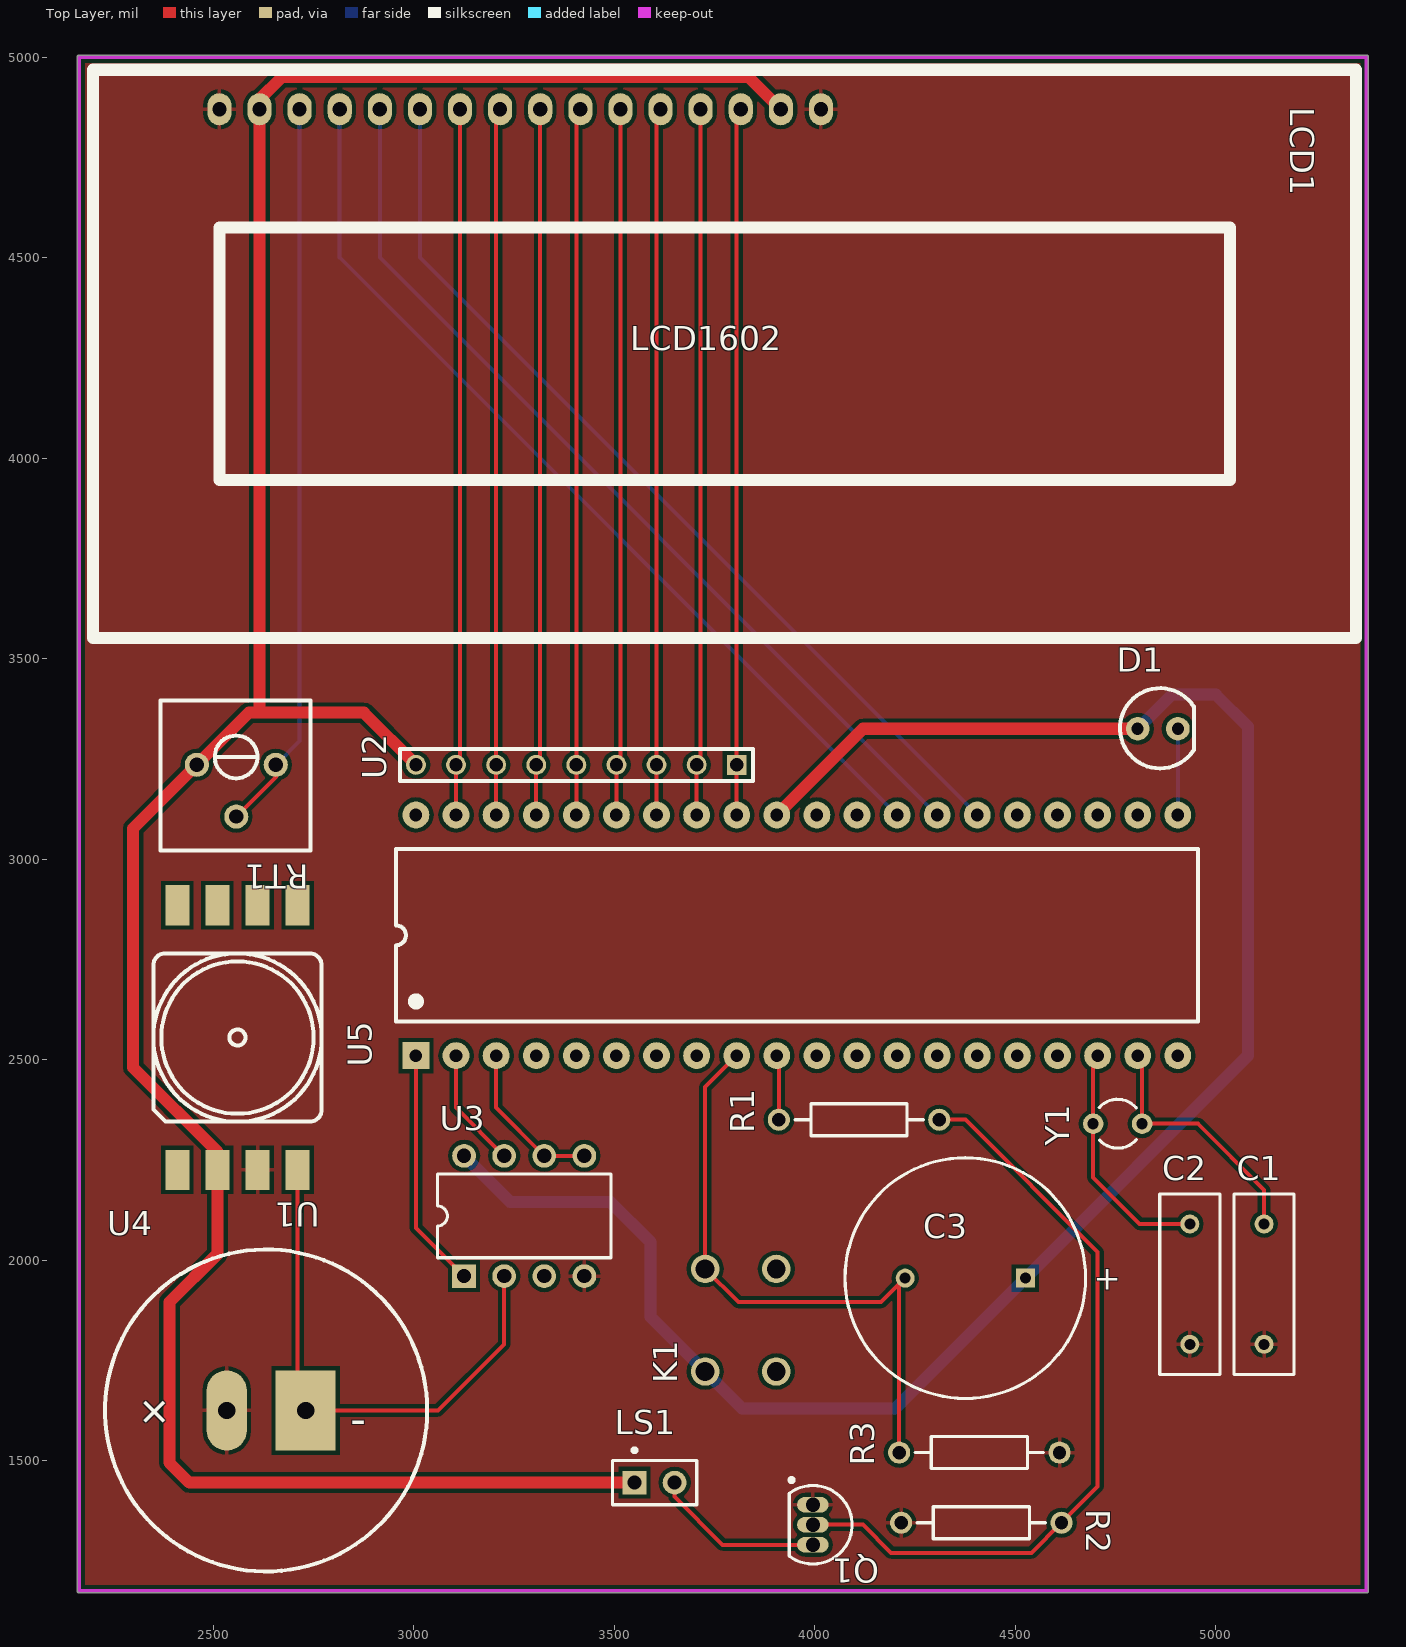
[diagram p0: Top Layer view]
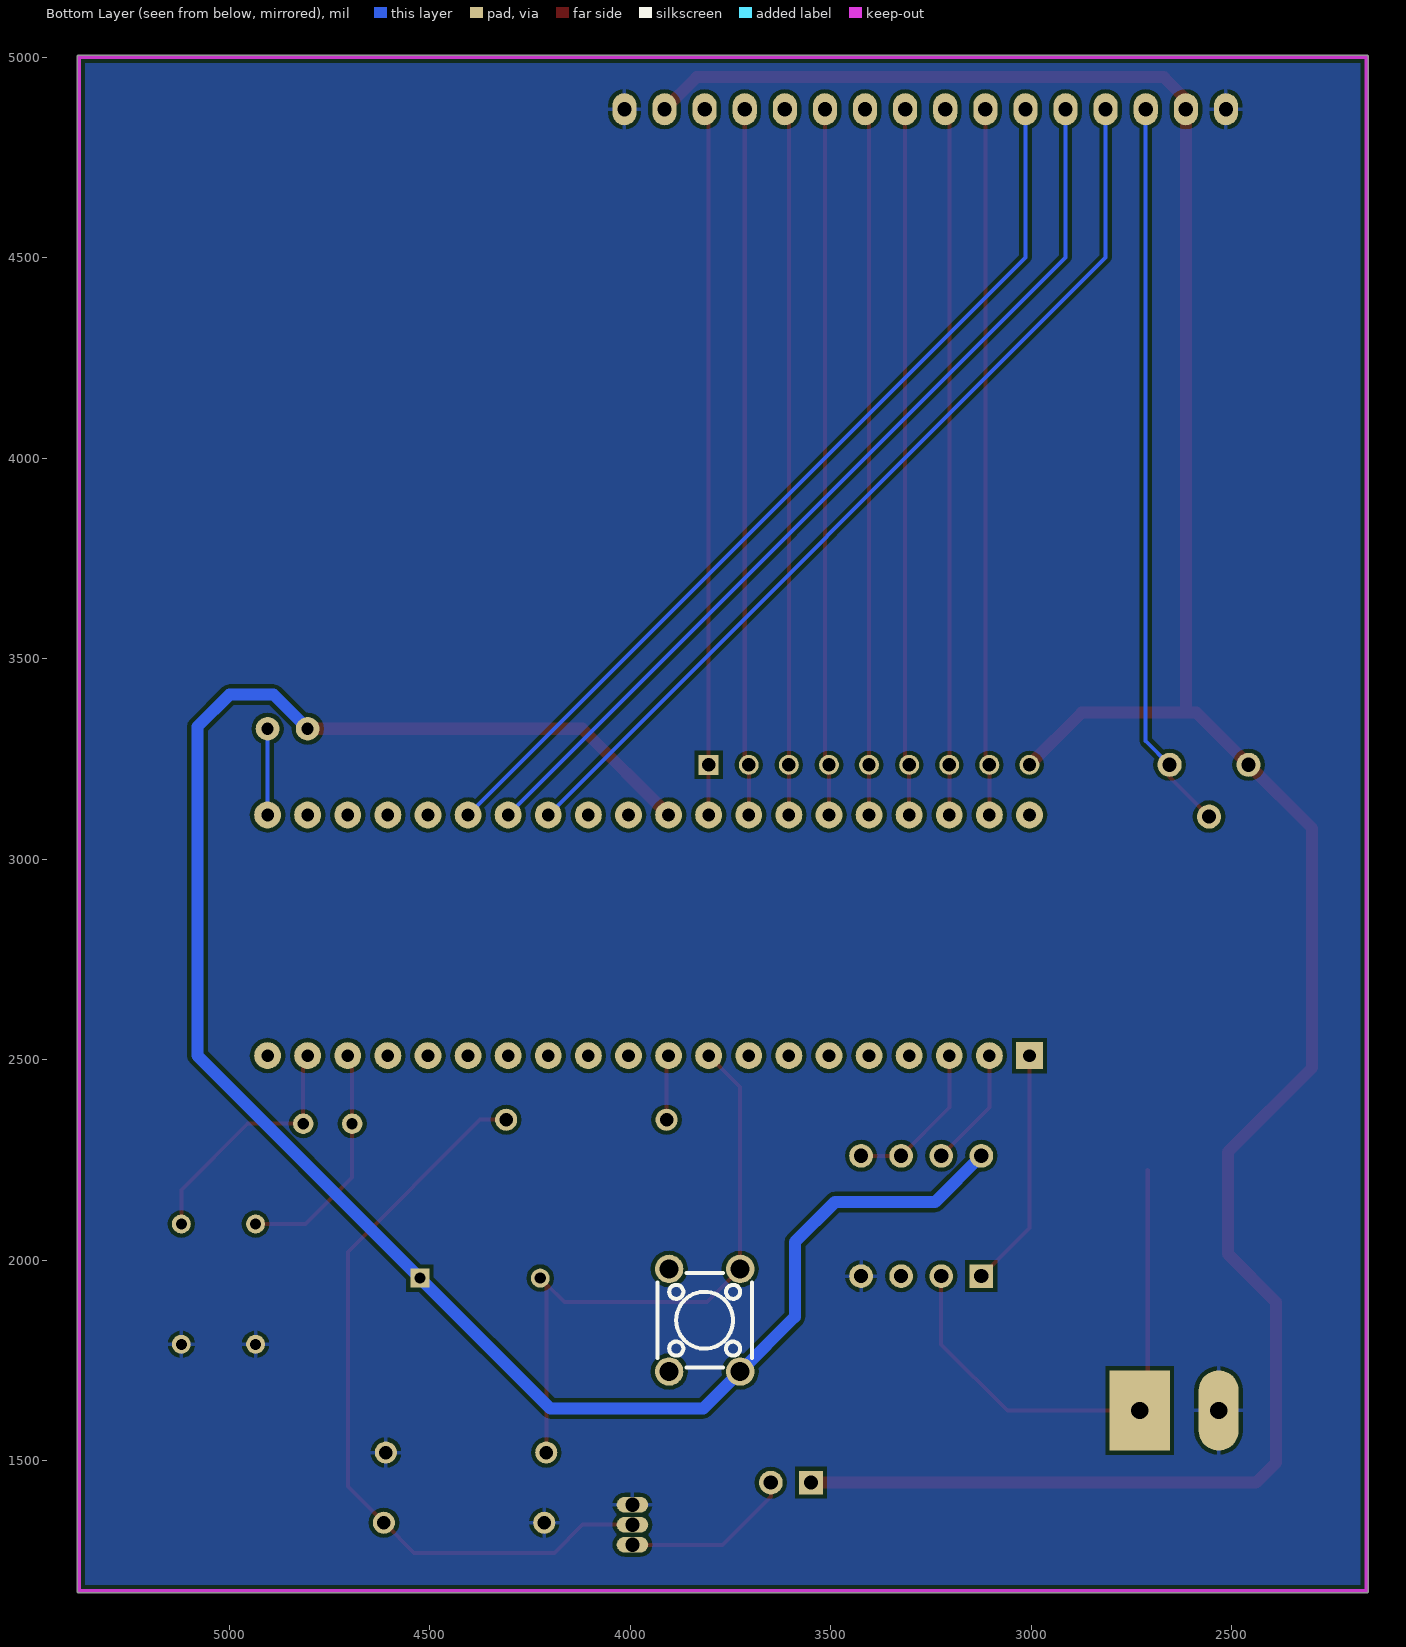
[diagram p1: Bottom Layer view, seen from below]
# Altium PCB MISC84281.PcbDoc
Units mil, origin at the board's own origin, x right, y up, seen from the top; angles counter-clockwise.
Board outline 3220.03 x 3835.03 mil, 2 copper layers (Top Layer, Bottom Layer); 18 components, 32 nets, 111 pads, 0 vias.

## Layer stack, top to bottom (the 12.6 mil dielectric is the usual default, probably not edited)
Top Solder: solder mask 0.4, Solder Resist, Dk 3.5
Top Layer: signal copper 1.4
Dielectric 1: dielectric 12.6, FR-4, Dk 4.8
Bottom Layer: signal copper 1.4
Bottom Solder: solder mask 0.4, Solder Resist, Dk 3.5

## Board outline
2159.99,1175 ccw(c2165,1175) 2165,1169.98 5375,1169.98 ccw(c5375,1175) 5380.02,1175 5380.02,5000 ccw(c5375,5000) 5375,5005.02 2165,5005.02 ccw(c2165,5000) 2159.99,5000

## Design rules (kind name [scope] priority, off if disabled: settings)
Clearance [All] p1: gap=10
MinimumSolderMaskSliver [All] p1: minsoldermaskwidth=0
PolygonConnect [All] p1: connectstyle=Relief reliefconductorwidth=10 reliefentries=4 polygonreliefangle="90 Angle" airgapwidth=10
RoutingVias [All] p1: holewidth=28 width=50 viastyle="Through Hole" minholewidth=28 minwidth=50 maxholewidth=28 maxwidth=50
SilkToSilkClearance [All] p1: silktosilkclearance=0
SilkToSolderMaskClearance [IsPad] p1: minsilkscreentomaskgap=0 clearancetoexposedcopper=TRUE
SolderMaskExpansion [All] p1: expansion=4
Width [All] p1: maxlimit=30 minlimit=10 preferedwidth=10
27 further rules are at their usual default settings.

## Components (designator, comment, footprint, x,y, rotation, side; value= is the part's Value field where it differs from the comment)
C1 "22U" RAD-0.3 5120,1940 r90 top
C2 "22U" RAD-0.3 4935,1940 r90 top
C3 "10UF" RB7.6-15 4375,1955 r0 top
D1 "LED" LED5-BLUE 4805,3325 r0 top
K1 "HH+" 四脚轻触开关 3815,1850 r90 top
LCD1 "LCD1602" LCD1602 2515,4870 r0 top
LS1 "Bell" PIN2 3550,1445 r0 top
Q1 "2N3904" TO-92A 3995,1340 r180 top
R1 "1K" AXIAL-0.4 4110,2350 r180 top
R2 "10K" AXIAL-0.4 4415,1345 r0 top
R3 "10K" AXIAL-0.4 4410,1520 r180 top
RT1 "10K" 电位器 2555,3220 r180 top
U1 "MPXA6115A6U" 482 2560,2555 r270 top
U2 "排阻" paizu 3405,3235 r180 top
U3 "ADC0832" P008 3275,2110 r0 top
U4 "Volts" "CAPACITANCE 1 FARAD 5,5 VOLT" 2631.58,1625 r0 top
U5 "AT89C52" DIP40 3955,2810 r90 top
Y1 "XTAL" R38 4755,2340 r90 top

## Footprints (in the part's own frame and the unit in brackets; to place one, negate y for a bottom-side part, rotate by r counter-clockwise, add the part's x,y. Pads: shape width x height; smd on the part's side, far side on the other; paste and mask are expansions set on the pad)
482 [mil]
  rect 100x60 smd paste+0 mask+2: 1(330,-150) 2(330,-50) 3(330,50) 4(330,150) 5(-330,150) 6(-330,50) 7(-330,-50) 8(-330,-150)
  silkscreen extent -210,-210 210,210
AXIAL-0.4 [mm] "Axial Device, Thru-Hole; 2 Leads; 0.4 in Pin Spacing"
  round 1.4 hole 0.85: 1(-5.08,0) 2(5.08,0)
  silkscreen extent -4.06,-1.02 4.06,1.02
"CAPACITANCE 1 FARAD 5,5 VOLT" [mil]
  rect 150x200 hole 43.31 paste+0 mask+2: 1(98.42,0)
  oval 100x200 hole 43.31 paste+0 mask+2: 2(-98.4,0)
  silkscreen extent -401,-402 402,402
DIP40 [mm]
  rect 1.7x1.7 hole 0.8: 1(-7.62,24.13)
  round 1.7 hole 0.8: 2(-7.62,21.59) 3(-7.62,19.05) 4(-7.62,16.51) 5(-7.62,13.97) 6(-7.62,11.43) 7(-7.62,8.89) 8(-7.62,6.35) 9(-7.62,3.81) 10(-7.62,1.27) 11(-7.62,-1.27) 12(-7.62,-3.81) 13(-7.62,-6.35) 14(-7.62,-8.89) 15(-7.62,-11.43) 16(-7.62,-13.97) 17(-7.62,-16.51) 18(-7.62,-19.05) 19(-7.62,-21.59) 20(-7.62,-24.13) 21(7.62,-24.13) 22(7.62,-21.59) 23(7.62,-19.05) 24(7.62,-16.51) 25(7.62,-13.97) 26(7.62,-11.43) 27(7.62,-8.89) 28(7.62,-6.35) 29(7.62,-3.81) 30(7.62,-1.27) 31(7.62,1.27) 32(7.62,3.81) 33(7.62,6.35) 34(7.62,8.89) 35(7.62,11.43) 36(7.62,13.97) 37(7.62,16.51) 38(7.62,19.05) 39(7.62,21.59) 40(7.62,24.13)
  silkscreen extent -5.46,-25.4 5.46,25.4, body extent -7.91,-26.19 7.65,26.16, height 4.7
LCD1602 [mil]
  oval 60x80 hole 35.43: 1(0,0) 2(100,0) 3(200,0) 4(300,0) 5(400,0) 6(500,0) 7(600,0) 8(700,0) 9(800,0) 10(900,0) 11(1000,0) 12(1100,0) 13(1200,0) 14(1300,0) 15(1400,0) 16(1500,0)
  silkscreen extent -315,-1319 2835,98, body extent -315,-1357 2854,80, height 414
LED5-BLUE [mm]
  round 1.5 hole 0.762: A(0,0) K(2.54,0)
  silkscreen extent -1.12,-2.51 3.56,2.57, body extent -1.58,-2.85 3.77,2.85, height 8.6
P008 [mm] "DIP; 8 Leads; Row Spacing 7.62 mm; Pitch 2.54 mm"
  rect 1.5x1.5 hole 0.9: 1(-3.81,-3.81)
  round 1.5 hole 0.9: 2(-1.27,-3.81) 3(1.27,-3.81) 4(3.81,-3.81) 5(3.81,3.81) 6(1.27,3.81) 7(-1.27,3.81) 8(-3.81,3.81)
  silkscreen extent -5.5,-2.65 5.5,2.65
paizu [mm]
  rect 1.26x1.26 hole 0.84 paste+0 mask+0.051: 1(-10.16,0)
  round 1.26 hole 0.84 paste+0 mask+0.051: 2(-7.62,0) 3(-5.08,0) 4(-2.54,0) 5(0,0) 6(2.54,0) 7(5.08,0) 8(7.62,0) 9(10.16,0)
  silkscreen extent -11.18,-1.02 11.18,1.02
PIN2 [mm] "Photosensitive Diode; 2 Leads"
  rect 1.5x1.5 hole 0.9: 1(0,0)
  round 1.5 hole 0.9: 2(2.54,0)
  silkscreen extent -1.4,-1.4 3.94,2.17
R38 [mm] "Crystal, Thru-Hole; 2 Leads; Body 3.1 x 8.2 mm (Dia.xH)"
  round 1.3 hole 0.7: 1(0,1.55) 2(0,-1.55)
  silkscreen extent -1.55,-1.19 1.55,1.17
RAD-0.3 [mm] "Radial Cap, Thru-Hole; 2 Leads; 0.3 in Pin Spacing"
  round 1.2 hole 0.7: 1(-3.81,0) 2(3.81,0)
  silkscreen extent -5.71,-1.91 5.71,1.91
RB7.6-15 [mm] "Polarized Capacitor (Radial); 2 Leads"
  rect 1.2x1.2 hole 0.7: 1(3.81,0)
  round 1.2 hole 0.7: 2(-3.81,0)
  silkscreen extent -7.62,-7.62 7.62,7.62
TO-92A [mm] "TO, Flat Index; 3 In-Line, Axial Leads; Body Dia. 4.5mm; Leads 0.51 x 0.48 mm (max)"
  oval 2x1 hole 0.9: 1(0,-1.27) 2(0,0) 3(0,1.27)
  silkscreen extent -2.48,-2.95 1.5,2.48, body extent -2.48,-2.5 1.5,2.5, height 6.86
四脚轻触开关 [mm]
  round 1.8 hole 1.2 paste+0 mask+0.102: 1(3.25,2.25) 2(-3.25,2.25) 3(3.25,-2.25) 4(-3.25,-2.25)
电位器 [mil]
  round 60 hole 35.43 paste+0 mask+2: 1(96.41,-15.12) 2(-2.01,114.1) 3(-100.44,-15.12)
  silkscreen extent -187,-175 187,199

## Part data
C1 C2: library part Cap, "Capacitor"
C3: library part "Cap Pol1", "Polarized Capacitor (Radial)"
K1: library part 四脚轻触开关
LS1: "Electrical Bell"
Q1: "NPN General Purpose Amplifier"
R1 R2 R3: library part Res2, "Resistor"
RT1: library part 电位器
U3: "U?"
U5: library part STC89C52
Y1: "Crystal Oscillator"

## Nets (pads, with @x,y where several pads share a name; then routed paths per layer and width w, separated by ;. In a path a pad name is that pad's centre, name@x,y a point inside that pad or via, vN(x,y) a via of type N, cw(c..) or ccw(c..) an arc to the next point about the centre after c; other vN are vias at no path point)
+5: C3.1 D1.A K1.2 U3.8 U5.31 | length 4842.1
  Top Layer w30: U5.31 4120,3325 D1.A
  Bottom Layer w30: U3.8 3240,2145 3490,2145 3590,2045 3590,1858.46 K1.2 3818.46,1630 4200,1630 C3.1 5080,2510 5080,3330 5000,3410 4890,3410 D1.A
GND: C1.1 C2.1 LCD1.1 LCD1.16 Q1.1 R2.1 R3.1 U1.3 U3.4 U4.2
NetC1_2: C1.2 U5.19 Y1.2 | length 631.9
  Top Layer w10: U5.19 4816.02,2498.98 Y1.2 4955,2340 5120,2175 C1.2
NetC2_2: C2.2 U5.18 Y1.1 | length 597.6
  Top Layer w10: U5.18 4693.98,2498.98 Y1.1 4693.98,2206.02 4810,2090 C2.2
NetC3_2: C3.2 K1.1 R3.2 U5.9 | length 1542.4
  Top Layer w10: U5.9 3726.42,2431.42 K1.1 3809.37,1895 4165,1895 C3.2@4210,1940 ; R3.2 C3.2@4210,1940 ; C3.2 C3.2@4210,1940
NetLCD1_3: LCD1.3 RT1.2 RT1.3 | length 1829.5
  Top Layer w10: RT1.2 2655.44,3204.33 RT1.3
  Bottom Layer w10: RT1.3 2715,3294.68 LCD1.3
NetLCD1_4: LCD1.4 U5.28 | length 2335.8
  Bottom Layer w10: LCD1.4 2815,4500 U5.28
NetLCD1_5: LCD1.5 U5.27 | length 2335.8
  Bottom Layer w10: LCD1.5 2915,4500 U5.27
NetLCD1_6: LCD1.6 U5.26 | length 2335.8
  Bottom Layer w10: LCD1.6 3015,4500 U5.26
NetLCD1_7: LCD1.7 U2.8 U5.39 | length 1764.1
  Top Layer w10: U5.39 U2.8 3115,3245 LCD1.7
NetLCD1_8: LCD1.8 U2.7 U5.38 | length 1764.1
  Top Layer w10: U5.38 U2.7 3205,4860 LCD1.8
NetLCD1_9: LCD1.9 U2.6 U5.37 | length 1764.1
  Top Layer w10: U5.37 U2.6 3315,3245 LCD1.9
NetLCD1_10: LCD1.10 U2.5 U5.36 | length 1764.1
  Top Layer w10: U5.36 U2.5 3405,4860 LCD1.10
NetLCD1_11: LCD1.11 U2.4 U5.35 | length 1764.1
  Top Layer w10: U5.35 U2.4 3515,3245 LCD1.11
NetLCD1_12: LCD1.12 U2.3 U5.34 | length 1764.1
  Top Layer w10: U5.34 U2.3 3605,4860 LCD1.12
NetLCD1_13: LCD1.13 U2.2 U5.33 | length 1764.1
  Top Layer w10: U5.33 U2.2 3715,3245 LCD1.13
NetLCD1_14: LCD1.14 U2.1 U5.32 | length 1764.1
  Top Layer w10: U5.32 U2.1 3805,4860 LCD1.14
NetLS1_2: LS1.2 Q1.3 | length 429.7
  Top Layer w10: LS1.2 3650,1410 3770,1290 Q1.3
NetQ1_2: Q1.2 R1.1 R2.2 | length 1924
  Top Layer w10: Q1.2 4120,1340 4190,1270 4540,1270 R2.2 4705,1435 4705,2020 4375,2350 R1.1
NetU1_4: U1.4 U3.2 U4.1 | length 1341.6
  Top Layer w10: U1.4 2710,1645 U4.1 3060,1625 3225,1790 U3.2
NetU3_1: U3.1 U5.1 | length 599.7
  Top Layer w10: U5.1 3005,2080 U3.1
NetU3_5: U3.5 U3.6 U5.3 | length 399.7
  Top Layer w10: U5.3 3205,2380 U3.6 U3.5
NetU3_7: U3.7 U5.2 | length 299.7
  Top Layer w10: U5.2 3105,2380 U3.7
P20: D1.K U5.21 | length 215
  Bottom Layer w10: U5.21 D1.K
P21: U5.22
P22: U5.23
P23: U5.24
P30: R1.2 U5.10 | length 162.1
  Top Layer w10: U5.10 3910,2505 R1.2
P31: U5.11
P32: U5.12
P33: U5.13
VCC: LCD1.2 LCD1.15 LS1.1 RT1.1 U1.2 U2.9 | length 6665.3
  Top Layer w30: U2.9 2875,3365 2620,3365 ; LS1.1 2440,1445 2390,1495 2390,1895 2510,2015 U1.2 2510,2270 2300,2480 2300,3076.53 RT1.1 2588.47,3365 2620,3365 ; LCD1.15 3835,4950 2670,4950 2615,4895 LCD1.2 2615,3370 2620,3365
pads on no net: K1.3 K1.4 U1.1 U1.5 U1.6 U1.7 U1.8 U3.3 U5.4 U5.5 U5.6 U5.7 U5.8 U5.14 U5.15 U5.16 U5.17 U5.20 U5.25 U5.29 U5.30 U5.40

## Polygon pours and split planes (outlines as drawn)
GND on Bottom Layer "G" (solid, remove dead copper, pour order 0): 1505,5160 1510,5165 6050,5165 6050,1410 5650,1010 5625,985 1915,985
GND on Top Layer "G" (solid, remove dead copper, pour order 4): 1030,900 1315,615 6690,615 6690,4810 5810,5690 5355,6145 1085,6145

## Keep-outs
Keep-Out Layer:
  lines w10: 5162.07,1175 5375,1175 5375,5000 2165,5000 2165,1175 5175,1175